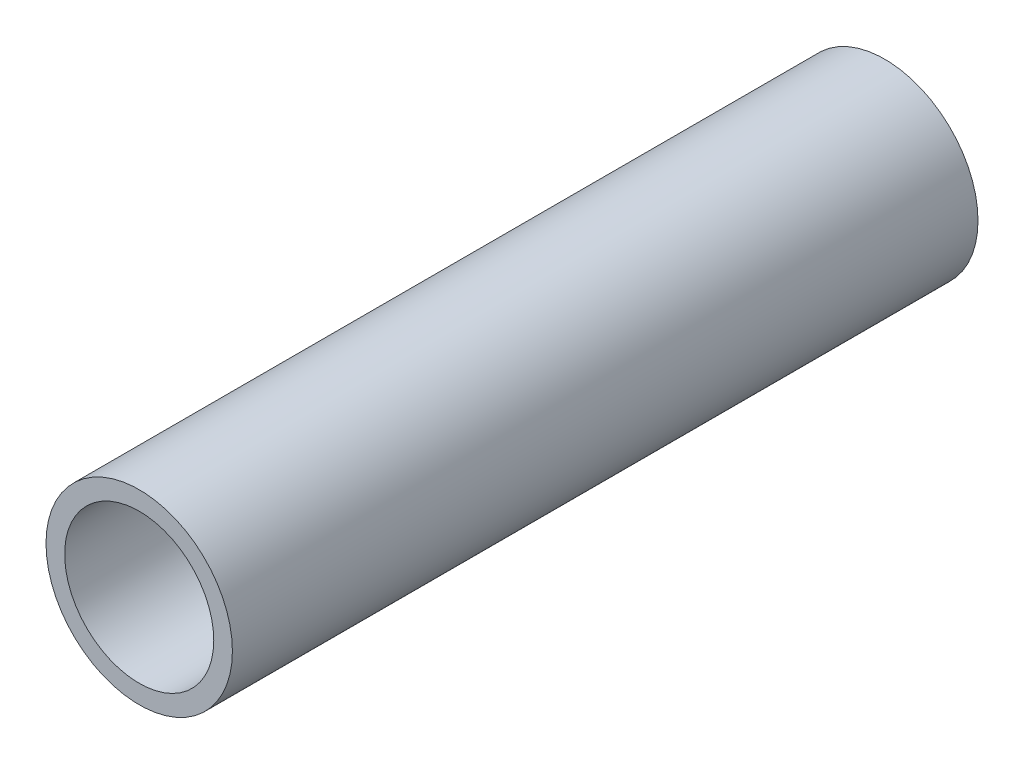
SolidWorks part; units mm, degrees
material "Q235-A"
ref_plane "前视基准面" through (0, 0, 0) normal (0, 0, 1) x (1, 0, 0)
ref_plane "上视基准面" through (0, 0, 0) normal (0, 1, 0) x (1, 0, 0)
ref_plane "右视基准面" through (0, 0, 0) normal (1, 0, 0) x (0, 0, -1)
sketch "草图1" plane through (0, 0, 0) normal (0, 0, 1) x (1, 0, 0)
  circle A0 centre (0, 0) radius 25
  circle A1 centre (0, 0) radius 20
  dimension "D1" = 5
  dimension "D2" = 50
extrude "凸台-拉伸1" add sketch "草图1" along normal blind 200
